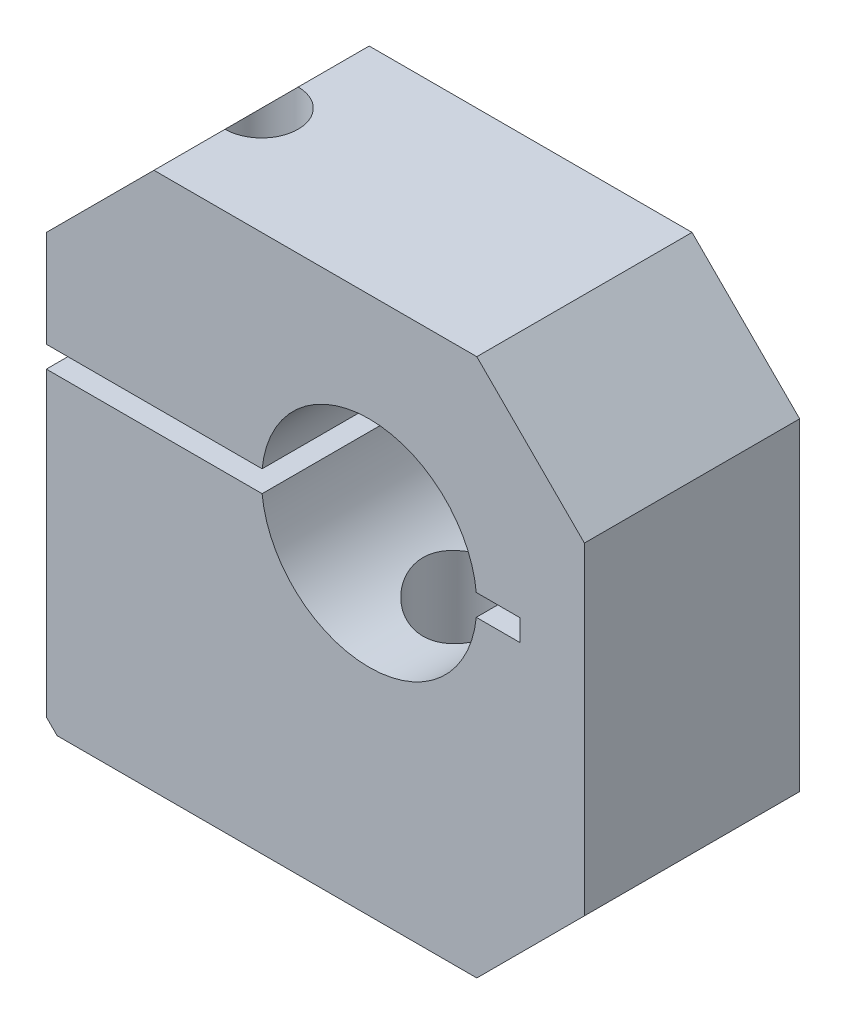
SolidWorks part; units mm, degrees
material "1023 碳钢板 (SS)"
ref_plane "前视基准面" through (0, 0, 0) normal (0, 0, 1) x (1, 0, 0)
ref_plane "上视基准面" through (0, 0, 0) normal (0, 1, 0) x (1, 0, 0)
ref_plane "右视基准面" through (0, 0, 0) normal (1, 0, 0) x (0, 0, -1)
sketch "草图1" plane through (0, 0, 0) normal (0, 0, 1) x (1, 0, 0)
  line L1 (-25, 25) -> (25, 25)
  line L2 (-25, 25) -> (-25, -25)
  line L3 (-25, -25) -> (25, -25)
  line L4 (25, 25) -> (25, -25)
  line L5 (-25, 25) -> (25, -25) construction
  line L6 (-25, -25) -> (25, 25) construction
  circle A0 centre (5, 5) radius 10
  point P0 (0, 0)
  dimension "D3" = 20
  dimension "D1" = 50
  dimension "D2" = 50
  dimension "D4" = 20
  dimension "D5" = 20
extrude "凸台-拉伸1" add sketch "草图1" along normal blind 20
chamfer "倒角1" distance 10 angle 45 3 edges at (25, -25, 10) (-25, 25, 10) (25, 25, 10)
chamfer "倒角2" distance 1 angle 45 1 edges at (-25, -25, 10)
sketch "草图2" plane through (0, 25, 0) normal (0, 1, 0) x (1, 0, 0)
  line L0 (-15, 0) -> (-15, -20) construction
  circle A0 centre (-15, -10) radius 4.1897
hole_wizard "M8 螺纹孔1" positions "草图3" profile "草图4" tap size "M8" standard "GB" end condition through all
sketch "草图3" plane through (0, 25, 0) normal (0, 1, 0) x (1, 0, 0)
  point P0 (-15, -10)
cosmetic thread "孔螺蚊线1" parameters "D2"=8
sketch "草图4" plane through (-15, 25, 10) normal (1, 0, 0) x (0, 0, 1)
  line L0 (0, 0) -> (0, 50)
  line L1 (0, 50) -> (3.4, 50)
  line L2 (3.4, 50) -> (3.4, 0)
  line L5 (3.4, 0) -> (0, 0)
  line L11 (0, -6.35) -> (0, 107.95) construction
  dimension "通孔螺纹孔钻头直径" = 6.8
  dimension "通孔螺纹孔钻头深度" = 50
sketch "草图5" plane through (0, -25, 0) normal (0, -1, 0) x (1, 0, 0)
  circle A0 centre (-15, 10) radius 4.5
  dimension "D1" = 9
extrude "切除-拉伸1" cut sketch "草图5" against normal blind 30
sketch "草图6" plane through (-25, 0, 0) normal (-1, 0, 0) x (0, 0, 1)
  line L0 (13.4, 25) -> (20, 25) construction
  line L1 (-7.2972, 6) -> (27.2972, 6)
  line L2 (-7.2972, 6) -> (-7.2972, 4)
  line L3 (-7.2972, 4) -> (27.2972, 4)
  line L4 (27.2972, 6) -> (27.2972, 4)
  line L5 (-7.2972, 6) -> (27.2972, 4) construction
  line L6 (-7.2972, 4) -> (27.2972, 6) construction
  point P0 (10, 5)
  dimension "D1" = 19
  dimension "D2" = 2
extrude "切除-拉伸2" cut sketch "草图6" against normal blind 44
sketch "草图7" plane through (0, -25, 0) normal (0, -1, 0) x (1, 0, 0)
  line L0 (25, 20) -> (25, 0) construction
  line L1 (-24, 20) -> (-24, 0) construction
  circle A0 centre (5, 10) radius 5
  point P7 (-24, 10)
  dimension "D2" = 10
  dimension "D1" = 20
extrude "切除-拉伸5" cut sketch "草图7" against normal blind 26
